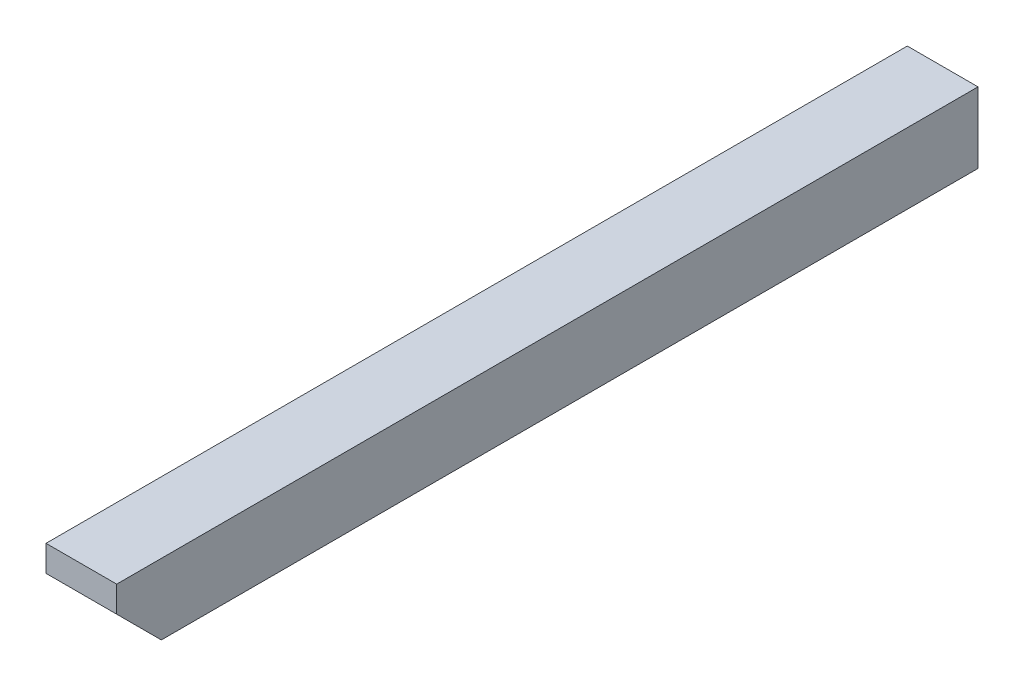
SolidWorks part; units mm, degrees
material "SS400B"
ref_plane "Front Plane" through (0, 0, 0) normal (0, 0, 1) x (1, 0, 0)
ref_plane "Top Plane" through (0, 0, 0) normal (0, 1, 0) x (1, 0, 0)
ref_plane "Right Plane" through (0, 0, 0) normal (1, 0, 0) x (0, 0, -1)
sketch "Sketch1" plane through (0, 0, 0) normal (0, 0, 1) x (1, 0, 0)
  line L1 (-9.5, 9.5) -> (9.5, 9.5)
  line L2 (-9.5, 9.5) -> (-9.5, -9.5)
  line L3 (-9.5, -9.5) -> (9.5, -9.5)
  line L4 (9.5, 9.5) -> (9.5, -9.5)
  line L5 (-9.5, 9.5) -> (9.5, -9.5) construction
  line L6 (-9.5, -9.5) -> (9.5, 9.5) construction
  point P0 (0, 0)
  dimension "D1" = 19
  dimension "D2" = 19
extrude "Boss-Extrude1" add sketch "Sketch1" along normal mid plane 231.5
chamfer "Chamfer1" distance 12 angle 45 1 edges at (0, -9.5, 115.75)
